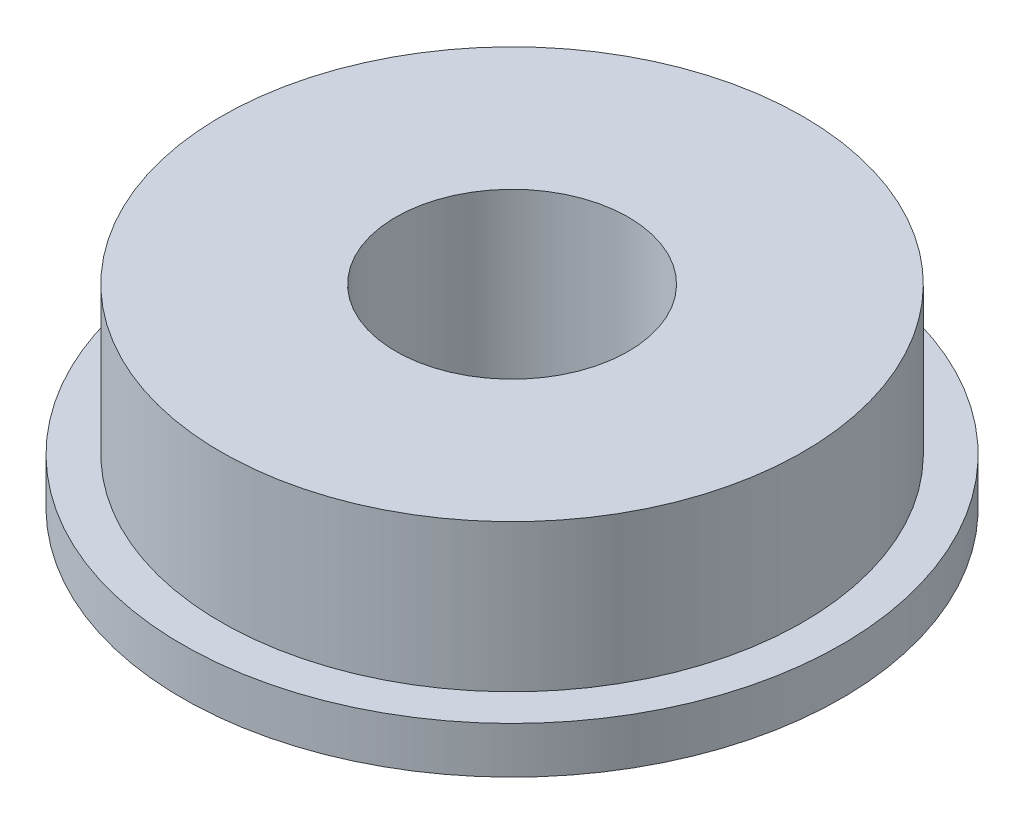
SolidWorks part; units mm, degrees
material "6061 合金"
ref_plane "前视基准面" through (0, 0, 0) normal (0, 0, 1) x (1, 0, 0)
ref_plane "上视基准面" through (0, 0, 0) normal (0, 1, 0) x (1, 0, 0)
ref_plane "右视基准面" through (0, 0, 0) normal (1, 0, 0) x (0, 0, -1)
sketch "草图1" plane through (0, 0, 0) normal (0, 0, 1) x (1, 0, 0)
  line L0 (0, 0) -> (0, 5185.6035) construction
  line L1 (3, 4.5991) -> (3, -0.4009)
  line L2 (3, -0.4009) -> (8.5, -0.4009)
  line L3 (8.5, -0.4009) -> (8.5, 0.7991)
  line L4 (8.5, 0.7991) -> (7.5, 0.7991)
  line L5 (7.5, 0.7991) -> (7.5, 4.5991)
  line L6 (7.5, 4.5991) -> (3, 4.5991)
  dimension "D1" = 3
  dimension "D2" = 5
  dimension "D3" = 4.5
  dimension "D4" = 3.8
  dimension "D5" = 1
revolve "旋转1" add sketch "草图1" angle 360 about L0
